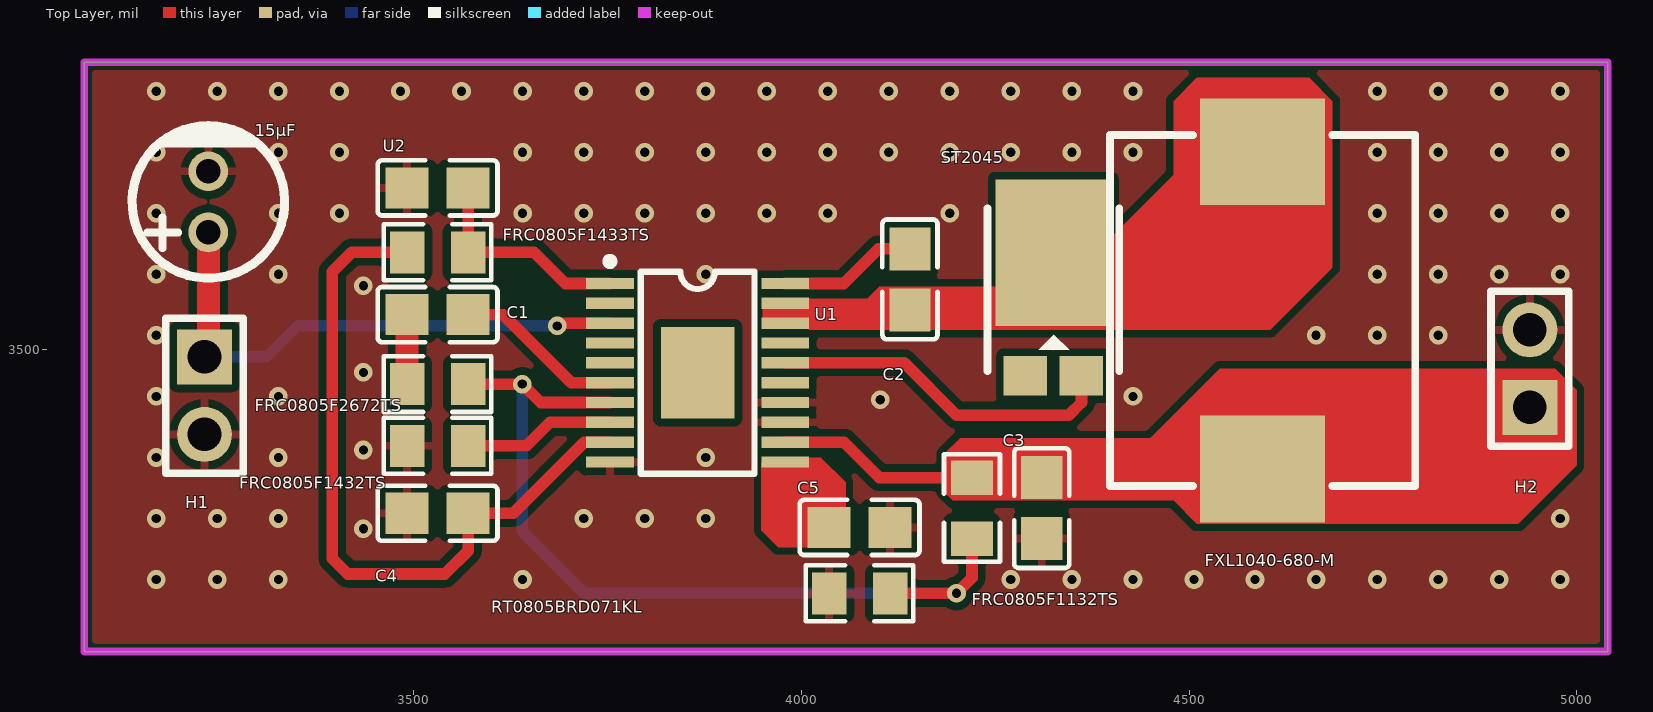
[diagram p0: Top Layer view]
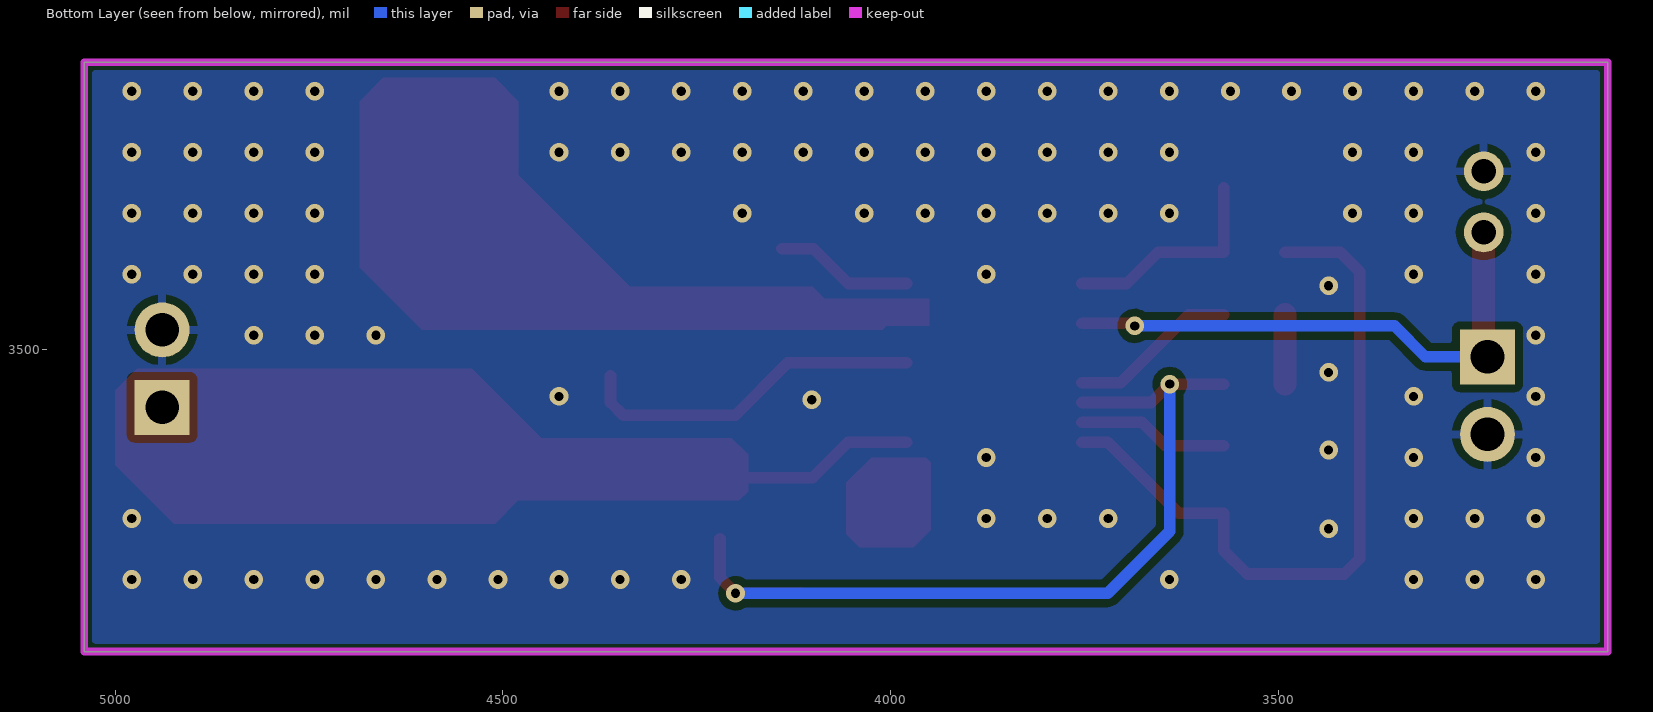
[diagram p1: Bottom Layer view, seen from below]
# Altium PCB MISC51833.pcbdoc
Units mil, origin at the board's own origin, x right, y up, seen from the top; angles counter-clockwise.
Board outline 1965 x 760 mil, 2 copper layers (Top Layer, Bottom Layer), stack 62.206 mil thick; 17 components, 13 nets, 54 pads, 99 vias.

## Layer stack, top to bottom
Top Solder Mask Layer: solder mask 0.394, Dk 3.3
Top Layer: signal copper 1.379
Dielectric1: surface 59.449, FR4, Dk 4.5
Bottom Layer: signal copper 1.378
Bottom Solder Mask Layer: solder mask 0.394, Dk 3.3

## Board outline
3075,3870 3075,3110 5040,3110 5040,3870

## Design rules (kind name [scope] priority, off if disabled: settings)
BoardOutlineClearance copperThickness2oz_1 [All] p2 off: genericclearance=7.99 ignorepadtopadclearanceinfootprint=FALSE except(0: Arc-SplitContinuation Track-SplitContinuation SMDPad-SplitContinuation THPad-SplitContinuation Via-SplitContinuation Fill-SplitContinuation Region-SplitContinuation Poly-SplitContinuation Text-SplitContinuation Hole-SplitContinuation; 5.98: Arc-CutoutEdge SMDPad-CutoutEdge THPad-CutoutEdge Via-CutoutEdge Fill-CutoutEdge Region-CutoutEdge Text-CutoutEdge; 6.93: Hole-OutlineEdge Hole-CutoutEdge; 10: Poly-OutlineEdge Poly-CutoutEdge; 11.81: Arc-OutlineEdge Track-OutlineEdge SMDPad-OutlineEdge THPad-OutlineEdge Via-OutlineEdge Fill-OutlineEdge Region-OutlineEdge Text-OutlineEdge Track-CutoutEdge)
BoardOutlineClearance copperThickness1oz_1 [All] p4: genericclearance=4.02 ignorepadtopadclearanceinfootprint=FALSE except(0: Arc-SplitContinuation Track-SplitContinuation SMDPad-SplitContinuation THPad-SplitContinuation Via-SplitContinuation Fill-SplitContinuation Region-SplitContinuation Poly-SplitContinuation Text-SplitContinuation Hole-SplitContinuation; 6: SMDPad-CutoutEdge THPad-CutoutEdge Via-CutoutEdge Fill-CutoutEdge Region-CutoutEdge Text-CutoutEdge; 6.93: Hole-OutlineEdge Hole-CutoutEdge; 10: Poly-OutlineEdge Poly-CutoutEdge; 11.8: Arc-OutlineEdge Track-OutlineEdge SMDPad-OutlineEdge THPad-OutlineEdge Via-OutlineEdge Fill-OutlineEdge Region-OutlineEdge Text-OutlineEdge; 11.81: Arc-CutoutEdge Track-CutoutEdge)
Clearance copperThickness2oz [All] p1 off: gap=7.99 ignorepadtopadclearanceinfootprint=FALSE except(5.98: SMDPad-Track SMDPad-SMDPad THPad-Track SMDPad-THPad THPad-THPad Track-Via SMDPad-Via THPad-Via Via-Via Fill-Track Region-Track Fill-SMDPad Region-SMDPad Fill-THPad Region-THPad Fill-Via Region-Via Fill-Fill Fill-Region Region-Region Arc-Track Arc-SMDPad Arc-THPad Arc-Via Fill-Arc Region-Arc Arc-Arc Text-Track SMDPad-Text Text-THPad Text-Via Fill-Text Region-Text Arc-Text Text-Text; 6.93: Hole-Track Hole-SMDPad Hole-THPad Hole-Via Fill-Hole Region-Hole Hole-Arc Hole-Text; 10: Poly-Track Poly-SMDPad Poly-THPad Poly-Via Poly-Fill Poly-Region Poly-Poly Poly-Arc Poly-Text Poly-Hole)
Clearance copperThickness1oz [All] p3: gap=4.02 ignorepadtopadclearanceinfootprint=FALSE except(5.98: SMDPad-Track SMDPad-SMDPad THPad-Track SMDPad-THPad THPad-THPad Track-Via SMDPad-Via THPad-Via Via-Via Fill-Track Region-Track Fill-SMDPad Region-SMDPad Fill-THPad Region-THPad Fill-Via Region-Via Fill-Fill Fill-Region Region-Region; 6: Arc-Track Arc-SMDPad Arc-THPad Arc-Via Fill-Arc Region-Arc Arc-Arc Text-Track SMDPad-Text Text-THPad Text-Via Fill-Text Region-Text Arc-Text Text-Text; 6.93: Hole-Track Hole-SMDPad Hole-THPad Hole-Via Fill-Hole Region-Hole Hole-Arc Hole-Text; 10: Poly-Track Poly-SMDPad Poly-THPad Poly-Via Poly-Fill Poly-Region Poly-Poly Poly-Arc Poly-Text Poly-Hole)
DiffPairsRouting differentialPair [All] p1: maxlimit=6 minlimit=6 mostfreqgap=6 toplayer_minwidth=5 toplayer_prefwidth=10 toplayer_maxwidth=100 toplayer_mingap=6 toplayer_prefgap=6 toplayer_maxgap=6 bottomlayer_minwidth=5 bottomlayer_prefwidth=10 bottomlayer_maxwidth=100 bottomlayer_mingap=6 bottomlayer_prefgap=6 bottomlayer_maxgap=6 maxuncoupledlength=10
HoleToHoleClearance otherClearance [All] p1: gap=11.81 allowstackedmicrovias=TRUE
Length netLength [All] p1: minlimit=0 maxlimit=0
MatchedLengths netLengthTolerance [All] p1: tolerance=1000
PasteMaskExpansion pasteMaskExpansion [All] p1: expansion=0
PlaneConnect innerPlane [All] p1: planeconnectstyle=Relief reliefexpansion=20 reliefentries=4 reliefconductorwidth=10 reliefairgap=10
PolygonConnect copperRegion [(InNet('GND'))] p1: connectstyle=Relief reliefconductorwidth=10 reliefentries=4 polygonreliefangle="90 Angle" airgapwidth=10 via.connectstyle=Relief via.reliefconductorwidth=10 via.reliefentries=4 via.polygonreliefangle="90 Angle" via.airgapwidth=10
RoutingVias viaSize [All] p1: holewidth=12.01 width=24.02 viastyle="Through Hole" minholewidth=11.81 minwidth=19.68 maxholewidth=248.03 maxwidth=393.7
SolderMaskExpansion solderMaskExpansion [IsVia] p1: expansion=-1000 istentingtop=TRUE
SolderMaskExpansion solderMaskExpansion [All] p2: expansion=2 istentingtop=FALSE
Width copperThickness2oz_2 [All] p1 off: maxlimit=100 minlimit=8 preferedwidth=10
Width copperThickness1oz_2 [All] p2: maxlimit=100 minlimit=5 preferedwidth=10

## Components (designator, comment, footprint, x,y, rotation, side; value= is the part's Value field where it differs from the comment)
15μF "LKMB1102A150MF" CAP-TH_BD5.0-P2.00-D0.8-FD 3235,3690 r90 top
C1 "CL21A106KAYNNNE" C0805 3530.65,3544.57 r180 top
C2 "CL21A106KAYNNNE" C0805 4140,3590 r90 top
C3 "CL21A106KAYNNNE" C0805 4310,3295 r270 top
C4 "FCC0805B681K500DT" C0805 3530.65,3288.28 r180 top
C5 "FM21X273K101ECG" C0805 4075,3270 r0 top
FRC0805F1132TS "" R0805 4220,3295 r270 top
FRC0805F1432TS "" R0805 3530.65,3375.37 r180 top
FRC0805F1433TS "" R0805 3530.65,3625 r180 top
FRC0805F2672TS "" R0805 3530.65,3455 r0 top
FXL1040-680-M "68μH" IND-SMD_L11.5-W10.0_104CDMCCDS 4595,3550 r270 top
H1 "" HDR-TH_2P-P2.54-V-M-1 3230,3440 r270 top
H2 "" HDR-TH_2P-P2.54-V-M-1 4939.69,3474.85 r90 top
RT0805BRD071KL "" R0805 4075,3185 r180 top
ST2045 "ST2045" TO-277_3P-L5.4-W4.0-LS6.5-BR 4325,3545 r270 top
U1 "LM5576MHX/NOPB" HTSSOP-20_L6.5-W4.4-P0.65-LS6.4-BL-EP3.0 3866.12,3469.57 r270 top
U2 "CL21B104KCFNNNE" C0805 3530.65,3708.01 r180 top

## Footprints (in the part's own frame and the unit in brackets; to place one, negate y for a bottom-side part, rotate by r counter-clockwise, add the part's x,y. Pads: shape width x height; smd on the part's side, far side on the other; paste and mask are expansions set on the pad)
C0805 [mm]
  rect 1.41x1.35 smd paste-100 mask+0.051: 1(-1,0) 2(1,0)
  silkscreen extent -1.96,-0.9 1.96,0.9
CAP-TH_BD5.0-P2.00-D0.8-FD [mm]
  round 1.3 hole 0.8: 1(-1,0) 2(1,0)
  silkscreen extent -2.5,-2.5 2.5,2.5
HDR-TH_2P-P2.54-V-M-1 [mm]
  rect 1.8x1.8 hole 1.1: 1(-1.27,0)
  round 1.8 hole 1.1: 2(1.27,0)
  silkscreen extent -2.54,-1.27 2.54,1.27
HTSSOP-20_L6.5-W4.4-P0.65-LS6.4-BL-EP3.0 [mil]
  rect 14.5x61.5 smd: 1(-115.16,-113) 2(-89.57,-113) 3(-63.98,-113) 4(-38.39,-113) 5(-12.8,-113) 6(12.79,-113) 7(38.39,-113) 8(63.98,-113) 9(89.57,-113) 10(115.16,-113) 11(115.16,113) 12(89.57,113) 13(63.98,113) 14(38.39,113) 15(12.79,113) 16(-12.8,113) 17(-38.39,113) 18(-63.98,113) 19(-89.57,113) 20(-115.16,113)
  rect 118.11x94.49 smd: 21(0,0)
  silkscreen extent -149,-118 130,73
IND-SMD_L11.5-W10.0_104CDMCCDS [mm]
  rect 3.5x4.1 smd: 1(-5.2,0) 2(5.2,0)
  silkscreen extent -5.75,-5 5.75,5
R0805 [mm]
  rect 1.133x1.377 smd paste-100 mask+0.051: 1(-1,0) 2(1,0)
  silkscreen extent -1.76,-0.92 1.76,0.92
TO-277_3P-L5.4-W4.0-LS6.5-BR [mm]
  rect 1.29x1.422 smd: 1(2.016,-0.92) 3(2.016,0.92)
  rect 4.8x3.8 smd: 2(-2.017,0)
  silkscreen extent -3.47,-2.16 1.86,2.16

## Via types
v1: diameter 24.02, hole 12, Top Layer to Bottom Layer, 99 vias

## Nets (pads, with @x,y where several pads share a name; then routed paths per layer and width w, separated by ;. In a path a pad name is that pad's centre, name@x,y a point inside that pad or via, vN(x,y) a via of type N, cw(c..) or ccw(c..) an arc to the next point about the centre after c; other vN are vias at no path point)
15V: C3.1 FRC0805F1132TS.1 FXL1040-680-M.2 H2.1 U1.12 | length 259.8
  Top Layer w15: U1.12 4055,3380 4100.63,3334.37 FRC0805F1132TS.1
$2N2: C1.1 U1.6 | length 219.5
  Top Layer w15: C1.1 3615.43,3544.57 3703.22,3456.78 U1.6
$2N3: C2.2 U1.20 | length 179.4
  Top Layer w15: U1.20 4054.73,3584.73 4099.37,3629.37 C2.2
$2N4: C2.1 FXL1040-680-M.1 ST2045.2 U1.18 U1.19
$2N5: ST2045.3 U1.16 | length 451.1
  Top Layer w15: U1.16 4132.63,3482.37 4200,3415 4345,3415 4361.22,3431.22 ST2045.3
$2N7: FRC0805F1433TS.1 U1.1 U2.1 | length 282.8
  Top Layer w15: U2.1 FRC0805F1433TS.1 3655,3625 3695.27,3584.73 U1.1
$2N8: FRC0805F1432TS.1 U1.8 | length 195.6
  Top Layer w15: FRC0805F1432TS.1 3645.37,3375.37 3675.59,3405.59 U1.8
$2N9: C4.1 FRC0805F1433TS.2 U1.9 | length 941.7
  Top Layer w15: FRC0805F1433TS.2 3420,3625 3395,3600 3395,3230 3415,3210 3540,3210 3570.02,3240.02 C4.1 3628.28,3288.28 3720,3380 U1.9
$2N10: FRC0805F1132TS.2 FRC0805F2672TS.2 RT0805BRD071KL.1 U1.7 | length 1140.6
  Top Layer w15: FRC0805F2672TS.2 v1(3640,3455) 3663.82,3431.18 U1.7 ; RT0805BRD071KL.1 v1(4200,3185) 4220,3205 FRC0805F1132TS.2
  Bottom Layer w15: v1(3640,3455) 3640,3265 3720,3185 v1(4200,3185)
$2N11: C5.1 U1.11
$2N13: C1.2 FRC0805F2672TS.1 | length 89.6
  Top Layer w30: FRC0805F2672TS.1 C1.2
$2N16: 15μF.1 H1.1 U1.3 | length 703.9
  Top Layer w15: v1(3685,3530) 3688.55,3533.55 U1.3
  Top Layer w30: H1.1 3235,3495 15μF.1
  Bottom Layer w15: H1.1 3310,3490 3350,3530 v1(3685,3530)
GND: 15μF.2 C3.2 C4.2 C5.2 FRC0805F1432TS.2 H1.2 H2.2 RT0805BRD071KL.2 U1.10 U1.13 U1.14 U2.2
  other v1: 3167.84,3202.84 3246.58,3202.84 3325.32,3202.84 3640.28,3202.84 4270.2,3202.84 4348.94,3202.84 4427.68,3202.84 4506.42,3202.84 4585.16,3202.84 4663.9,3202.84 4742.64,3202.84 4821.38,3202.84 4900.12,3202.84 4978.86,3202.84 3435,3268.24 3167.84,3281.58 3246.58,3281.58 3325.32,3281.58 3719.02,3281.58 3797.76,3281.58 3876.5,3281.58 4978.86,3281.58 3167.84,3360.32 3325.32,3360.32 3876.5,3360.32 3435,3370 4101.57,3434.71 3167.84,3439.06 3325.32,3439.06 4427.68,3439.06 3435,3470 3167.84,3517.8 4663.9,3517.8 4742.64,3517.8 4821.38,3517.8 3435,3581.66 3167.84,3596.54 3325.32,3596.54 3876.5,3596.54 4742.64,3596.54 4821.38,3596.54 4900.12,3596.54 4978.86,3596.54 3167.84,3675.28 3325.32,3675.28 3404.06,3675.28 3640.28,3675.28 3719.02,3675.28 3797.76,3675.28 3876.5,3675.28 3955.24,3675.28 4033.98,3675.28 4191.46,3675.28 4742.64,3675.28 4821.38,3675.28 4900.12,3675.28 4978.86,3675.28 3167.84,3754.02 3325.32,3754.02 3404.06,3754.02 3640.28,3754.02 3719.02,3754.02 3797.76,3754.02 3876.5,3754.02 3955.24,3754.02 4033.98,3754.02 4112.72,3754.02 4191.46,3754.02 4270.2,3754.02 4348.94,3754.02 4427.68,3754.02 4742.64,3754.02 4821.38,3754.02 4900.12,3754.02 4978.86,3754.02 3167.84,3832.76 3246.58,3832.76 3325.32,3832.76 3404.06,3832.76 3482.8,3832.76 3561.54,3832.76 3640.28,3832.76 3719.02,3832.76 3797.76,3832.76 3876.5,3832.76 3955.24,3832.76 4033.98,3832.76 4112.72,3832.76 4191.46,3832.76 4270.2,3832.76 4348.94,3832.76 4427.68,3832.76 4742.64,3832.76 4821.38,3832.76 4900.12,3832.76 4978.86,3832.76
pads on no net: ST2045.1 U1.2 U1.4 U1.5 U1.15 U1.17 U1.21

## Polygon pours and split planes (outlines as drawn)
GND on Top Layer (solid, remove dead copper, pour order 0): 3000,3995 3000,3000 5210,3000 5210,3995
GND on Bottom Layer (solid, remove dead copper, pour order 2): 3010,3965 3010,3025 5105,3025 5105,3965

## Keep-outs
Board Outline Layer:
  the board outline again, w10

## Other copper
Top Layer:
  region net $2N4: 3950,3530 3950,3565 4085,3565 4100.55,3580.55 4335.55,3580.55 4480,3725 4480,3820 4510,3850 4655,3850 4685,3820 4685,3605 4605,3525 4010,3525 4005,3530
  region net $2N11: 3948.29,3354.41 3953.88,3360 4025,3360 4056.89,3328.11 4056.89,3261.34 4040.36,3244.8 3970.2,3244.8 3948.29,3266.71
  region net 15V: 4183.89,3364.34 4204.56,3385 4450,3385 4539.85,3474.85 4972.28,3474.85 5000,3447.13 5000,3350 4925,3275 4510,3275 4480,3305 4195,3305 4183.89,3316.11